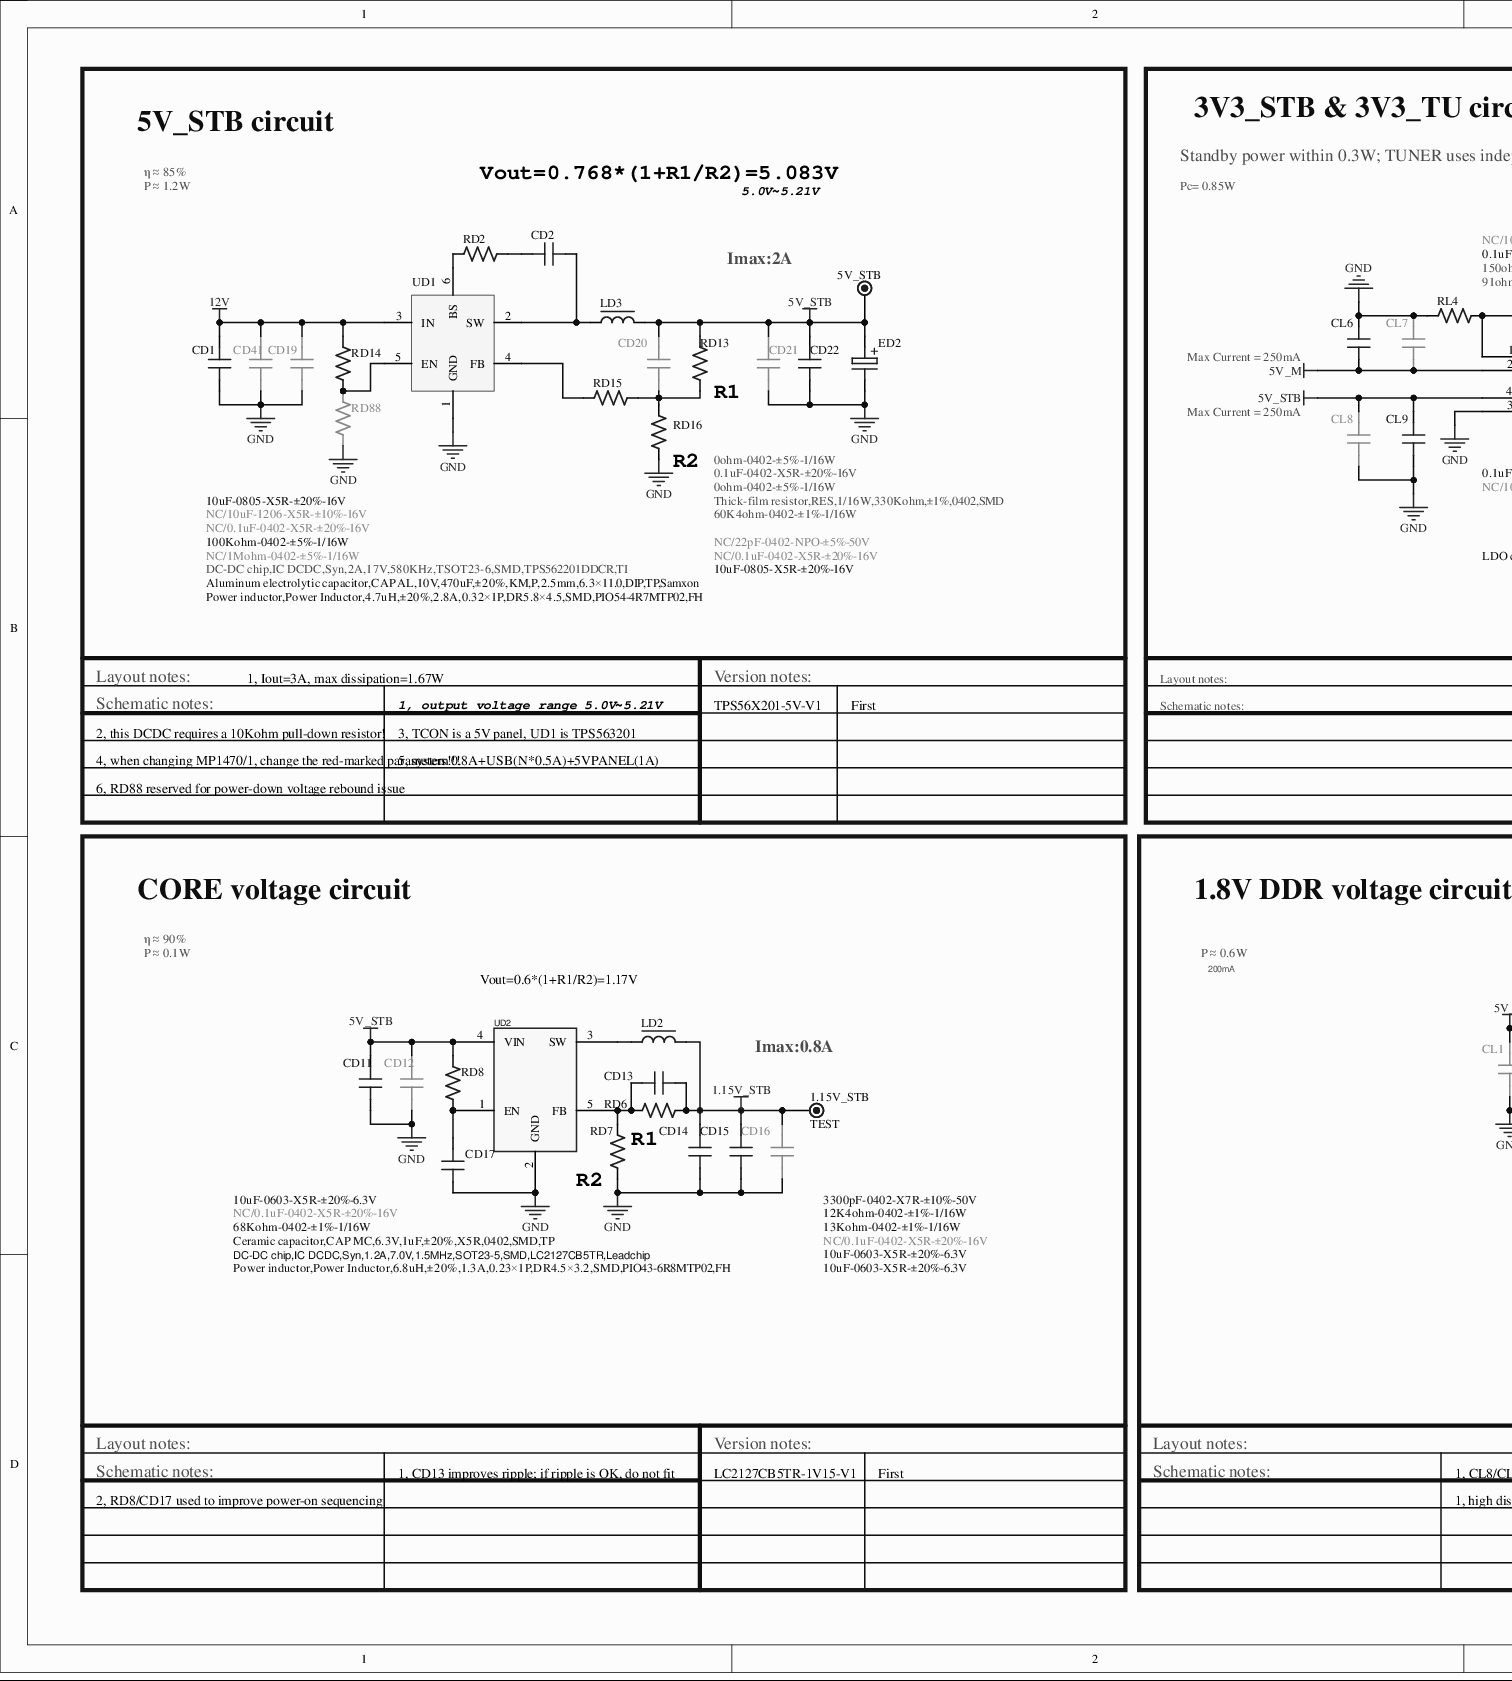
[diagram p0: MISC84438-7.SchDoc, left]
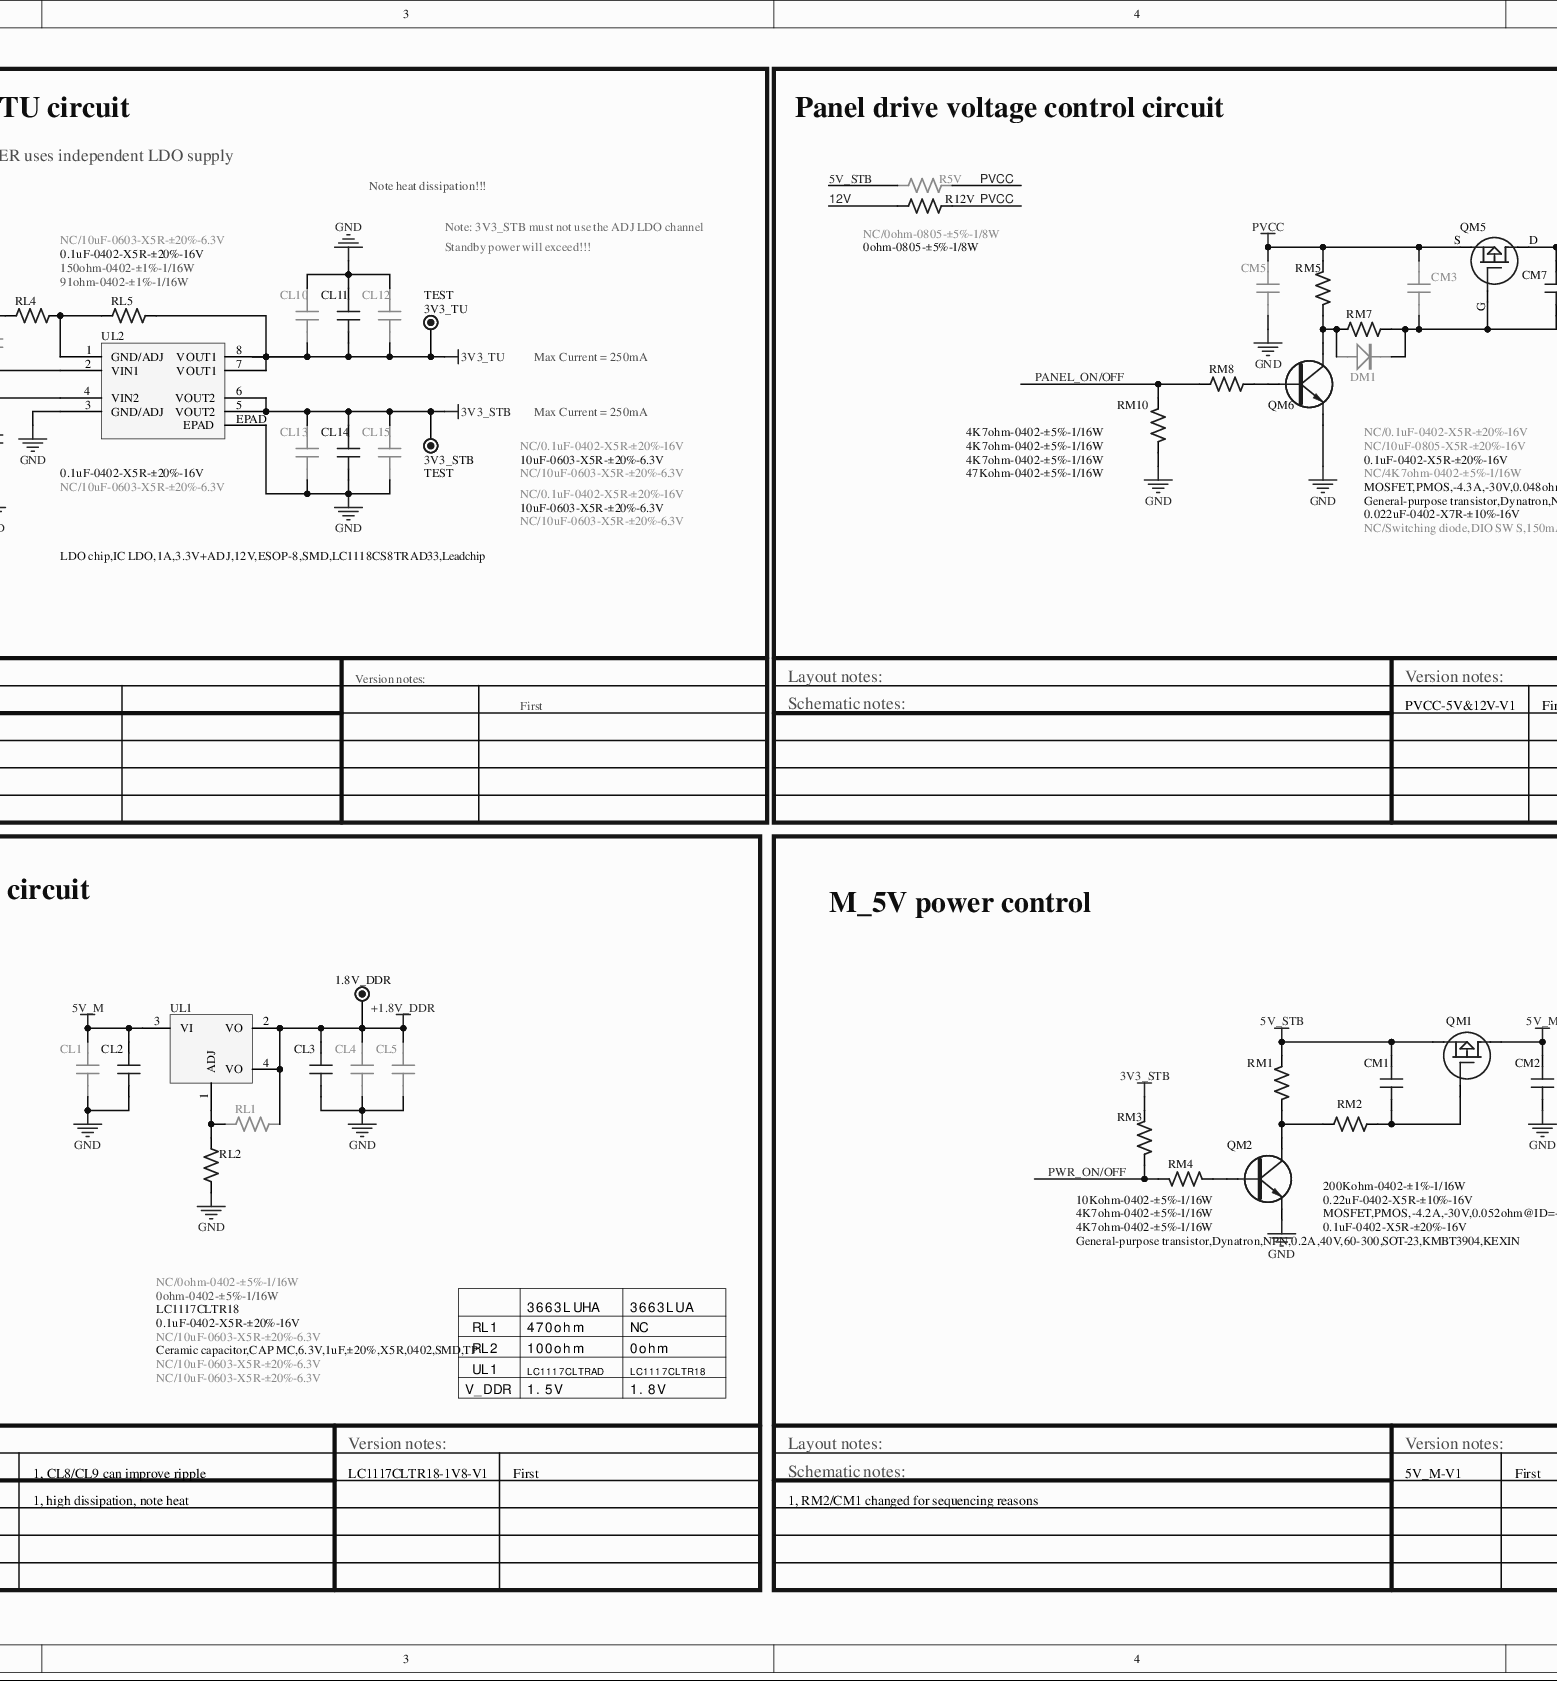
[diagram p1: MISC84438-7.SchDoc, middle]
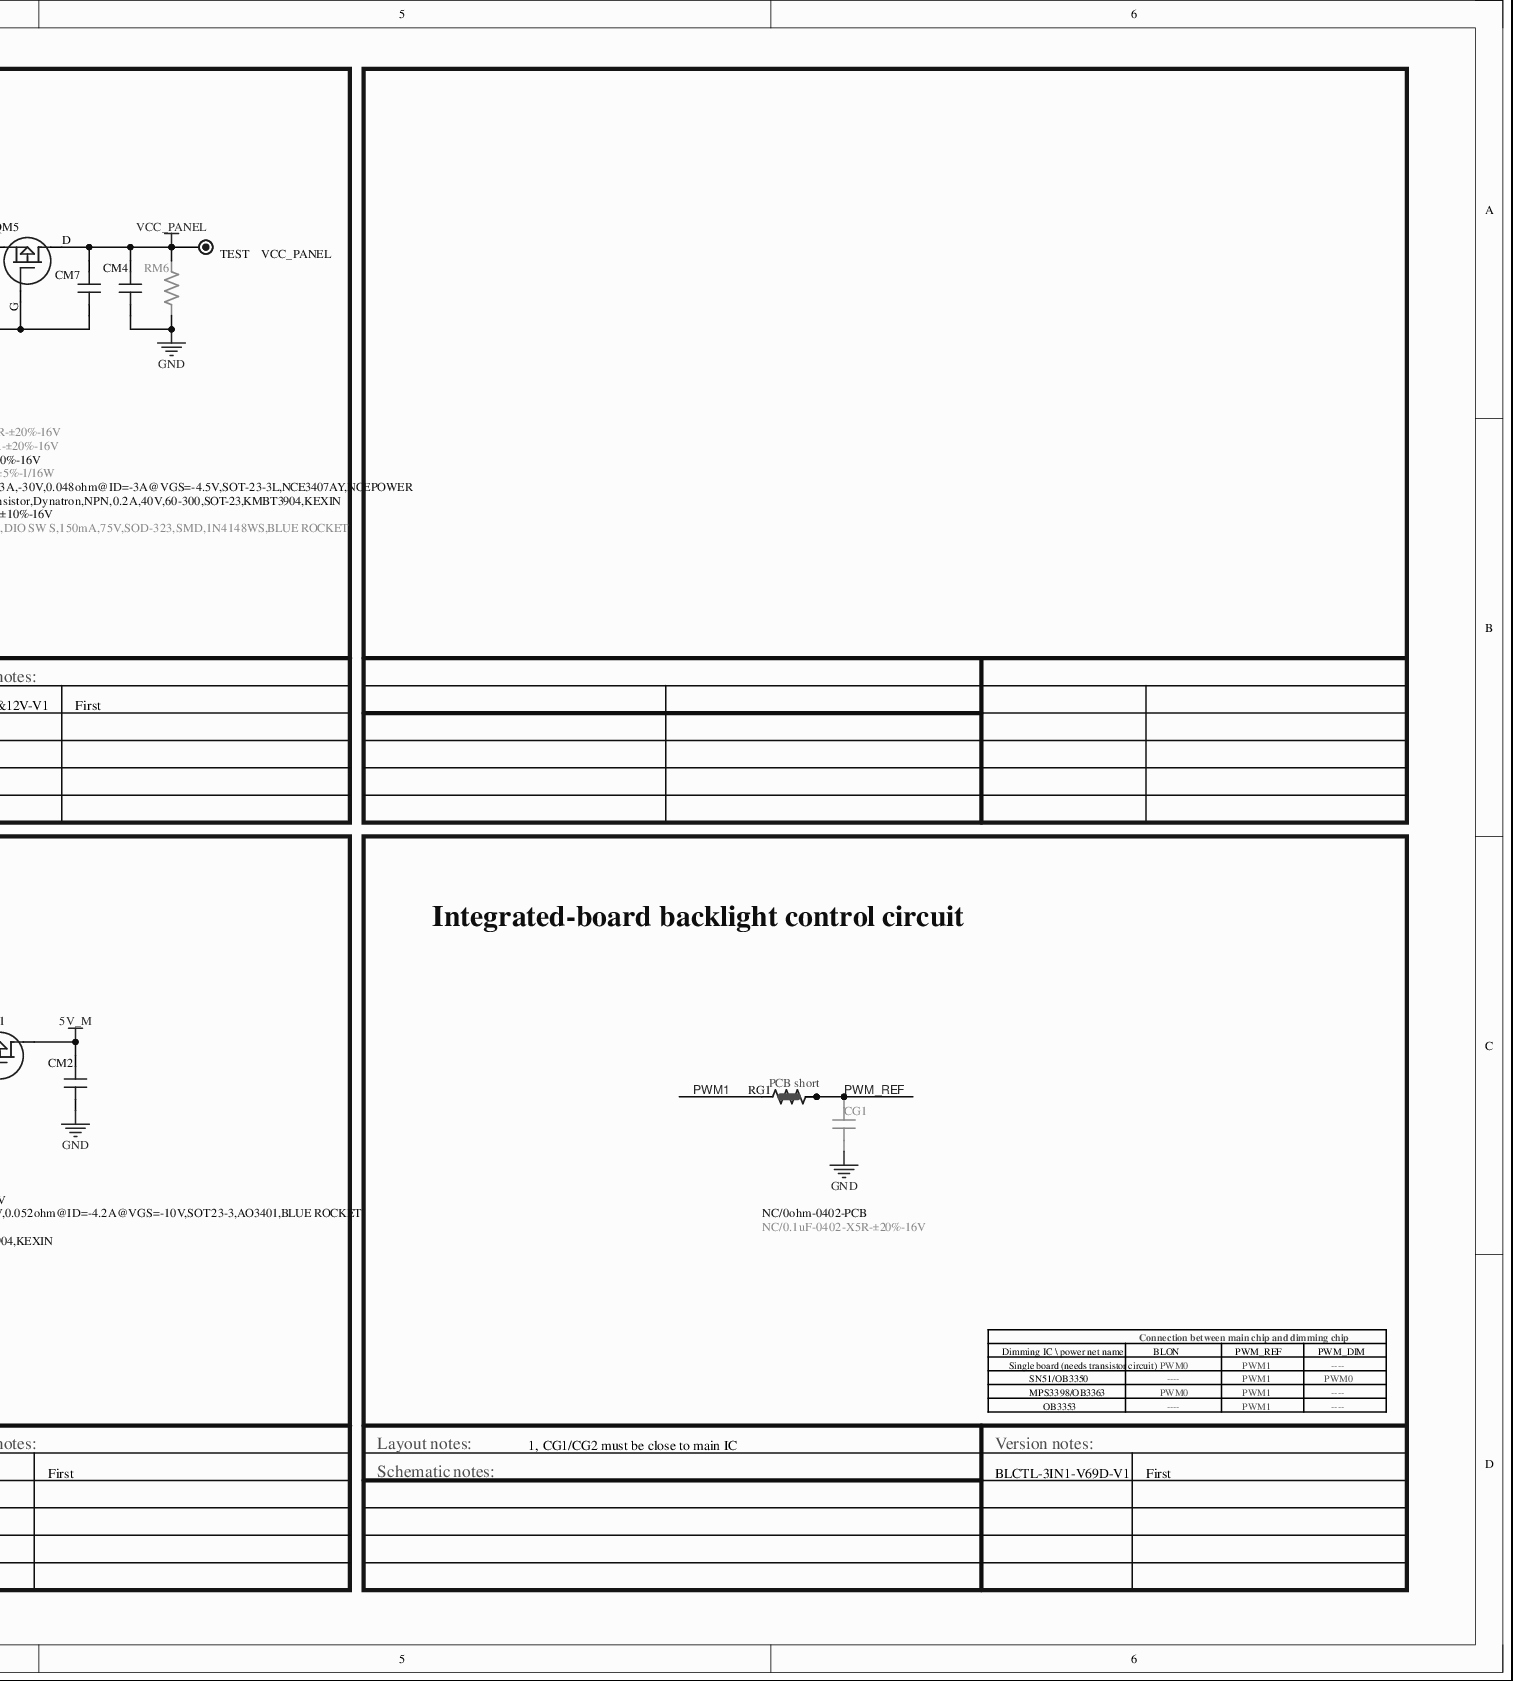
[diagram p2: MISC84438-7.SchDoc, right]
# Altium project MISC84438-18.PrjPCB (part 3 of 8)

## Sheet MISC84438-7.SchDoc
size 812 x 309 mm

### Parts
1.8V_DDR  TEST  [TP]  (value not drawn)
1.15V_STB  TEST  [TP]
3V3_STB  TEST  [TP]
3V3_TU  TEST  [TP]
5V_STB  TEST  [TP]  (value not drawn)
CD1  10uF-0805-X5R-±20%-16V  [C0805]
CD2  0.1uF-0402-X5R-±20%-16V  [C0402]
CD11  10uF-0603-X5R-±20%-6.3V  [C0603]
CD12  NC/0.1uF-0402-X5R-±20%-16V  [C0402]
CD13  3300pF-0402-X7R-±10%-50V  [C0402]
CD14  10uF-0603-X5R-±20%-6.3V  [C0603]
CD15  10uF-0603-X5R-±20%-6.3V  [C0603]
CD16  NC/0.1uF-0402-X5R-±20%-16V  [C0402]
CD17  Ceramic capacitor,CAP MC,6.3V,1uF,±20%,X5R,0402,SMD,TP  [C0402]
CD19  NC/0.1uF-0402-X5R-±20%-16V  [C0402]
CD20  NC/22pF-0402-NPO-±5%-50V  [C0402]
CD21  NC/0.1uF-0402-X5R-±20%-16V  [C0402]
CD22  10uF-0805-X5R-±20%-16V  [C0805]
CD41  NC/10uF-1206-X5R-±10%-16V  [C1206]
CG1  NC/0.1uF-0402-X5R-±20%-16V  [C0402]
CL1  NC/10uF-0603-X5R-±20%-6.3V  [C0603]
CL2  0.1uF-0402-X5R-±20%-16V  [C0402]
CL3  Ceramic capacitor,CAP MC,6.3V,1uF,±20%,X5R,0402,SMD,TP  [C0402]
CL4  NC/10uF-0603-X5R-±20%-6.3V  [C0603]
CL5  NC/10uF-0603-X5R-±20%-6.3V  [C0603]
CL6  0.1uF-0402-X5R-±20%-16V  [C0402]
CL7  NC/10uF-0603-X5R-±20%-6.3V  [C0603]
CL8  NC/10uF-0603-X5R-±20%-6.3V  [C0603]
CL9  0.1uF-0402-X5R-±20%-16V  [C0402]
CL10  NC/0.1uF-0402-X5R-±20%-16V  [C0402]
CL11  10uF-0603-X5R-±20%-6.3V  [C0603]
CL12  NC/10uF-0603-X5R-±20%-6.3V  [C0603]
CL13  NC/0.1uF-0402-X5R-±20%-16V  [C0402]
CL14  10uF-0603-X5R-±20%-6.3V  [C0603]
CL15  NC/10uF-0603-X5R-±20%-6.3V  [C0603]
CM1  0.22uF-0402-X5R-±10%-16V  [C0402]
CM2  0.1uF-0402-X5R-±20%-16V  [C0402]
CM3  NC/0.1uF-0402-X5R-±20%-16V  [C0402]
CM4  0.1uF-0402-X5R-±20%-16V  [C0402]
CM5  NC/10uF-0805-X5R-±20%-16V  [C0805]
CM7  0.022uF-0402-X7R-±10%-16V  [C0402]
DM1  NC/Switching diode,DIO SW S,150mA,75V,SOD-323,SMD,1N4148WS,BLUE ROCKET  [DIODE-S-12]
ED2  Aluminum electrolytic capacitor,CAP AL,10V,470uF,±20%,KM,P,2.5mm,6.3×11.0,DIP,TP,Samxon  [EC(6.3*11)-V-2.5]
LD2  Power inductor,Power Inductor,6.8uH,±20%,1.3A,0.23×1P,DR4.5×3.2,SMD,PIO43-6R8MTP02,FH  [L(4.5*3.5)-S]
LD3  Power inductor,Power Inductor,4.7uH,±20%,2.8A,0.32×1P,DR5.8×4.5,SMD,PIO54-4R7MTP02,FH  [L(6.0*4.5)-S]
QM1  MOSFET,PMOS,-4.2A,-30V,0.052ohm@ID=-4.2A@VGS=-10V,SOT23-3,AO3401,BLUE ROCKET  [SOT-23-1]
QM2  General-purpose transistor,Dynatron,NPN,0.2A,40V,60-300,SOT-23,KMBT3904,KEXIN  [SOT-23]
QM5  MOSFET,PMOS,-4.3A,-30V,0.048ohm@ID=-3A@VGS=-4.5V,SOT-23-3L,NCE3407AY,NCEPOWER  [SOT-23-1]
QM6  General-purpose transistor,Dynatron,NPN,0.2A,40V,60-300,SOT-23,KMBT3904,KEXIN  [SOT-23]
R5V  NC/0ohm-0805-±5%-1/8W  [R0805]
R12V  0ohm-0805-±5%-1/8W  [R0805]
RD2  0ohm-0402-±5%-1/16W  [R0402]
RD6  12K4ohm-0402-±1%-1/16W  [R0402]
RD7  13Kohm-0402-±1%-1/16W  [R0402]
RD8  68Kohm-0402-±1%-1/16W  [R0402]
RD13  Thick-film resistor,RES,1/16W,330Kohm,±1%,0402,SMD  [R0402]
RD14  100Kohm-0402-±5%-1/16W  [R0402]
RD15  0ohm-0402-±5%-1/16W  [R0402]
RD16  60K4ohm-0402-±1%-1/16W  [R0402]
RD88  NC/1Mohm-0402-±5%-1/16W  [R0402]
RG1  NC/0ohm-0402-PCB  [R0402SC]
RL1  NC/0ohm-0402-±5%-1/16W  [R0402]
RL2  0ohm-0402-±5%-1/16W  [R0402]
RL4  150ohm-0402-±1%-1/16W  [R0402]
RL5  91ohm-0402-±1%-1/16W  [R0402]
RM1  4K7ohm-0402-±5%-1/16W  [R0402]
RM2  200Kohm-0402-±1%-1/16W  [R0402]
RM3  10Kohm-0402-±5%-1/16W  [R0402]
RM4  4K7ohm-0402-±5%-1/16W  [R0402]
RM5  4K7ohm-0402-±5%-1/16W  [R0402]
RM6  NC/4K7ohm-0402-±5%-1/16W  [R0402]
RM7  47Kohm-0402-±5%-1/16W  [R0402]
RM8  4K7ohm-0402-±5%-1/16W  [R0402]
RM10  4K7ohm-0402-±5%-1/16W  [R0402]
UD1  DC-DC chip,IC DCDC,Syn,2A,17V,580KHz,TSOT23-6,SMD,TPS562201DDCR,TI  [SOT-23-6]
UD2  DC-DC chip,IC DCDC,Syn,1.2A,7.0V,1.5MHz,SOT23-5,SMD,LC2127CB5TR,Leadchip  [SOT-23-5]
UL1  LC1117CLTR18  [SOT-223]
UL2  LDO chip,IC LDO,1A,3.3V+ADJ,12V,ESOP-8,SMD,LC1118CS8TRAD33,Leadchip  [SOP8/1.27-3]
VCC_PANEL  TEST  [TP]

### Blocks framed on the sheet
5V_STB circuit: 5V_STB CD1 CD2 CD19-CD22 CD41 ED2 LD3 RD2 RD13-RD16 RD88 UD1
3V3_STB & 3V3_TU circuit: 3V3_STB 3V3_TU CL6-CL15 RL4 RL5 UL2
Panel drive voltage control circuit: CM3-CM5 CM7 DM1 QM5 QM6 R5V R12V RM5-RM8 RM10 VCC_PANEL
CORE voltage circuit: 1.15V_STB CD11-CD17 LD2 RD6-RD8 UD2
1.8V DDR voltage circuit: 1.8V_DDR CL1-CL5 RL1 RL2 UL1
M_5V power control: CM1 CM2 QM1 QM2 RM1-RM4
Integrated-board backlight control circuit: CG1 RG1

### Nets
1.15V_STB: 1.15V_STB.1 CD13.1 CD14.2 CD15.2 CD16.2 LD2.2 RD6.2
3V3_STB: 3V3_STB.1 CL13.1 CL14.1 CL15.2 RM3.1 UL2.5(VOUT2) UL2.6(VOUT2)
3V3_TU: 3V3_TU.1 CL10.2 CL11.1 CL12.1 RL5.2 UL2.7(VOUT1) UL2.8(VOUT1)
5V_M: CL1.2 CL2.2 CL6.2 CL7.2 CM2.1 QM1.D UL1.3(VI) UL2.2(VIN1)
5V_STB: 5V_STB.1 CD11.2 CD12.1 CD20.1 CD21.1 CD22.1 CL8.2 CL9.2 CM1.1 ED2.1 LD3.2 QM1.S R5V.1 RD8.1 RD13.2 RM1.2 UD2.4(VIN) UL2.4(VIN2)
12V: CD1.1 CD19.1 CD41.2 R12V.1 RD14.1 UD1.3(IN)
+1.8V_DDR: 1.8V_DDR.1 CL3.2 CL4.2 CL5.2 RL1.1 UL1.2(VO) UL1.4(VO)
GND: CD1.2 CD11.1 CD12.2 CD14.1 CD15.1 CD16.1 CD17.1 CD19.2 CD21.2 CD22.2 CD41.1 CG1.2 CL1.1 CL2.1 CL3.1 CL4.1 CL5.1 CL6.1 CL7.1 CL8.1 CL9.1 CL10.1 CL11.2 CL12.2 CL13.2 CL14.2 CL15.1 CM2.2 CM4.2 CM5.1 ED2.2 QM2.E QM6.E RD7.1 RD16.1 RD88.1 RL2.2 RL4.1 RM6.2 RM10.2 UD1.1(GND) UD2.2(GND) UL2.3(GND/ADJ) UL2.EPAD
PVCC: CM3.2 CM5.2 QM5.S R5V.2 R12V.2 RM5.2
PWM_REF: CG1.1 RG1.2 RG1.3
VCC_PANEL: CM4.1 CM7.2 QM5.D RM6.1 VCC_PANEL.1
PANEL_ON/OFF: RM8.1 RM10.1
PWM1: RG1.1
PWR_ON/OFF: RM3.2 RM4.2
NetCD2_1: CD2.1 RD2.2
NetCD2_2: CD2.2 LD3.1 UD1.2(SW)
NetCD13_2: CD13.2 RD6.1 RD7.2 UD2.5(FB)
NetCD17_2: CD17.2 RD8.2 UD2.1(EN)
NetCD20_2: CD20.2 RD13.1 RD15.2 RD16.2
NetCM1_2: CM1.2 QM1.G RM2.2
NetCM3_1: CM3.1 CM7.1 DM1.K QM5.G RM7.2
NetDM1_A: DM1.A QM6.C RM5.1 RM7.1
NetLD2_1: LD2.1 UD2.3(SW)
NetQM2_B: QM2.B RM4.1
NetQM2_C: QM2.C RM1.1 RM2.1
NetQM6_B: QM6.B RM8.2
NetRD2_1: RD2.1 UD1.6(BS)
NetRD14_2: RD14.2 RD88.2 UD1.5(EN)
NetRD15_1: RD15.1 UD1.4(FB)
NetRL1_2: RL1.2 RL2.1 UL1.1(ADJ)
NetRL4_2: RL4.2 RL5.1 UL2.1(GND/ADJ)

### Notes on the sheet
- η ≈ 85%
- P ≈ 1.2W
- Vout=0.768*(1+R1/R2)=5.083V
- 5.0V~5.21V
- Standby power within 0.3W; TUNER uses independent LDO supply
- Pc= 0.85W
- Note heat dissipation!!!
- Note: 3V3_STB must not use the ADJ LDO channel
- Standby power will exceed!!!
- Imax:2A
- Max Current = 250mA
- (near RD16) R2
- (near RD13) R1
- Layout notes:
- Schematic notes:
- 2, this DCDC requires a 10Kohm pull-down resistor!
- 1, Iout=3A, max dissipation=1.67W
- 1, output voltage range 5.0V~5.21V
- 3, TCON is a 5V panel, UD1 is TPS563201
- Version notes:
- TPS56X201-5V-V1
- First
- PVCC-5V&12V-V1
- 4, when changing MP1470/1, change the red-marked parameters!!!
- 6, RD88 reserved for power-down voltage rebound issue
- 5, system 0.8A+USB(N*0.5A)+5VPANEL(1A)
- η ≈ 90%
- P ≈ 0.1W
- Vout=0.6*(1+R1/R2)=1.17V
- P ≈ 0.6W
- 200mA
- Imax:0.8A
- R1
- R2
- RL1
- RL2
- 3663LUHA
- 470ohm
- 100ohm
- 3663LUA
- NC
- 0ohm
- Dimming IC \ power net name
- Connection between main chip and dimming chip
- BLON
- PWM_REF
- PWM_DIM
- V_DDR
- UL1
- LC1117CLTRAD
- 1.5V
- LC1117CLTR18
- 1.8V
- Single board (needs transistor circuit)
- SN51/OB3350
- MPS3398/OB3363
- OB3353
- PWM0
- ----
- PWM1
- 1, CD13 improves ripple; if ripple is OK, do not fit
- LC2127CB5TR-1V15-V1
- 1, CL8/CL9 can improve ripple
- LC1117CLTR18-1V8-V1
- 5V_M-V1
- 1, CG1/CG2 must be close to main IC
- BLCTL-3IN1-V69D-V1
- 2, RD8/CD17 used to improve power-on sequencing
- 1, high dissipation, note heat
- 1, RM2/CM1 changed for sequencing reasons

### Library data of the parts
CD1 CD22 CM5 = 10uF-0805-X5R-±20%-16V-D
CD2 = 0.1uF-0402-X7R-±10%-16V-D
CD11 CD14 CD15 CL1 CL4 CL5 CL7 CL8 CL11 CL12 CL14 CL15 = 10uF-0603-X5R-±20%-6.3V-D
CD12 CD16 CG1 CL2 CL3 CM1 CM2 CM4 = 0.1uF-0402-Y5V-+80%-20%-16V-D
CD13 = 3300pF-0402-X7R-±10%-50V-D
CD17 = 1uF-0402-X5R-±20%-16V-D
CD19 CD21 CL6 CL9 CL10 CL13 CM3 = 0.1uF-0402-X5R-±20%-16V-D
CD20 = 22pF-0402-NPO-±5%-50V-D
CD41 = 10uF-1206-X5R-±10%-16V-D
CM7 = 0.022uF-0402-X7R-±10%-16V-D
DM1 = 1N4148WS-D
ED2 = 470uF-10V-±20%-6.3×11-105℃-黑底白字-编带-F=2.5-XF-DHAI: Electrolytic
LD2 = SLN43T-6R8M-D
LD3 = SWPA6045S4R7MT-D
QM1 = WPM2341A-3/TR-D
QM2 QM6 = LMBT3904LT1G-D-NPN: Q-NPN-#-#-#
QM5 = WPM3407C-3/TR-D
R5V R12V = 0ohm-0805-±5%-1/8W-D
RD2 RD15 RL1 RL2 = 0ohm-0402-±5%-1/16W-D
RD6 = 12Kohm-0402-±1%-1/16W-D
RD7 = 12K4ohm-0402-±1%-1/16W-D
RD8 = 68Kohm-0402-±1%-1/16W-D
RD13 = 39Kohm-0402-±1%-1/16W-D: RES
RD14 RM2 = 100Kohm-0402-±5%-1/16W-D
RD16 = 6K8ohm-0402-±1%-1/16W-D
RD88 = 1Mohm-0402-±5%-1/16W-D
RG1 = 0ohm-0402-PCB-D
RL4 = 150ohm-0402-±1%-1/16W-D
RL5 = 91ohm-0402-±1%-1/16W-D
RM1 RM5 RM6 RM8 = 4k7ohm-0402-±5%-1/16W-D
RM3 RM4 = 10Kohm-0402-±5%-1/16W-D
RM7 = 47Kohm-0402-±5%-1/16W-D
RM10 = 2K2ohm-0402-±5%-1/16W-D
UD1 = DC-DC芯片,IC DCDC,Syn,3A,17V,650kHz,SOT-23,SMD,SN1501019DDCR,TI-D
UD2 = DC-DC芯片,IC DCDC,Syn,1.2A,7.0V,1.5MHz,SOT23-5,SMD,LC2127CB5TR,Leadchip-D
UL1 = LC1117CLTR18-D
UL2 = LC1118-D